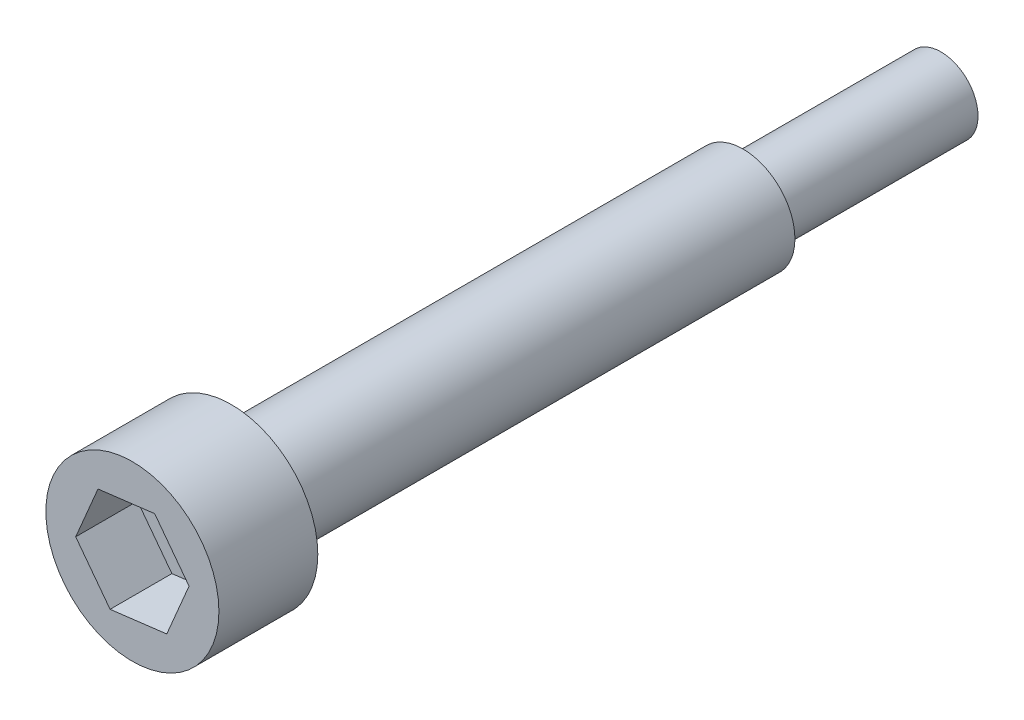
from build123d import *

# Parameters (mm, degrees)
SKETCH_1_R          = 7
EXTRUDE_1_DEPTH     = 8
SKETCH_2_R          = 4.191
EXTRUDE_2_DEPTH     = 41.4
SKETCH_3_R          = 3
EXTRUDE_3_DEPTH     = 16
CUT_EXTRUDE_1_DEPTH = 5


with BuildPart() as part:
    # 草图1 → 凸台-拉伸1 (new body)
    with BuildSketch(Plane.XY):
        with Locations((-26.159273046, -76.997288483)):
            Circle(SKETCH_1_R)
    extrude(amount=EXTRUDE_1_DEPTH)

    # 草图2 → 凸台-拉伸2 (add)
    with BuildSketch(Plane(origin=(0, 0, 0), x_dir=(-1, 0, 0), z_dir=(0, 0, -1))):
        with Locations(Location((26.159273046, -76.997288483, 0), (0, 0, 180))):
            Circle(SKETCH_2_R)
    extrude(amount=EXTRUDE_2_DEPTH)

    # 草图3 → 凸台-拉伸3 (add)
    with BuildSketch(Plane(origin=(0, 0, -41.4), x_dir=(-1, 0, 0), z_dir=(0, 0, -1))):
        with Locations(Location((26.159273046, -76.997288483, 0), (0, 0, 180))):
            Circle(SKETCH_3_R)
    extrude(amount=EXTRUDE_3_DEPTH)

    # 草图4 → 切除-拉伸1 (cut)
    with BuildSketch(Plane.XY.offset(8)):
        Polygon((-24.356132828, -72.744992787), (-28.940299035, -73.309575399), (-30.743439252, -77.561871096), (-27.962413264, -81.249584179), (-23.378247058, -80.685001566), (-21.57510684, -76.43270587), align=None)
    extrude(amount=-CUT_EXTRUDE_1_DEPTH, mode=Mode.SUBTRACT)


solid = part.part
